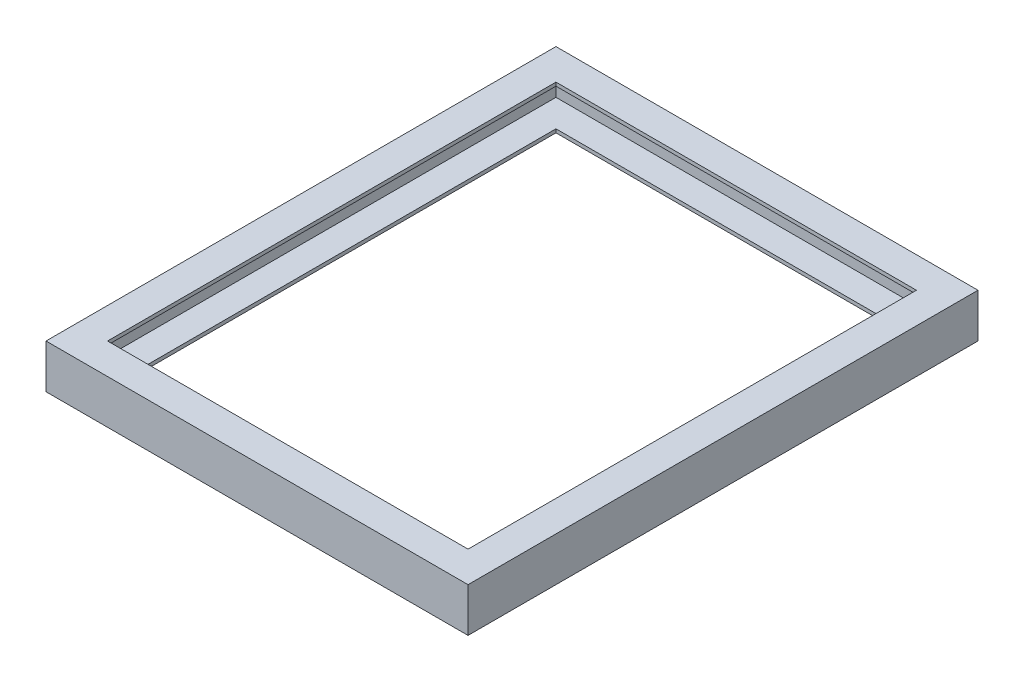
from build123d import *

# Parameters (mm, degrees)
BOSS_EXTRUDE1_DEPTH = 580
BOSS_EXTRUDE2_DEPTH = 472
BOSS_EXTRUDE3_DEPTH = 580


with BuildPart() as part:
    # Sketch1 → Boss-Extrude1 (new body)
    with BuildSketch(Plane.XY):
        Polygon((-10.73531847, 12.748914521), (-45.73531847, 12.748914521), (-45.73531847, -37.251085479), (-10.73531847, -37.251085479), (-10.73531847, -33.251085479), (-41.73531847, -33.251085479), (-41.73531847, 8.748914521), (-10.73531847, 8.748914521), align=None)
    extrude(amount=BOSS_EXTRUDE1_DEPTH)

    # Sketch2 → Boss-Extrude2 (add)
    with BuildSketch(Plane(origin=(-41.73531847, 0, 0), x_dir=(0, 0, -1), z_dir=(1, 0, 0))):
        Polygon((-545, 12.748914521), (-580, 12.748914521), (-580, -37.251085479), (-545, -37.251085479), (-545, -33.251085479), (-576, -33.251085479), (-576, 8.748914521), (-545, 8.748914521), align=None)
        Polygon((-35, -33.251085479), (-35, -37.251085479), (0, -37.251085479), (0, 12.748914521), (-35, 12.748914521), (-35, 8.748914521), (-4, 8.748914521), (-4, -33.251085479), align=None)
    extrude(amount=BOSS_EXTRUDE2_DEPTH)

    # Sketch3 → Boss-Extrude3 (add)
    with BuildSketch(Plane.XY.offset(580)):
        Polygon((399.26468153, 12.748914521), (434.26468153, 12.748914521), (434.26468153, -37.251085479), (399.26468153, -37.251085479), (399.26468153, -33.251085479), (430.26468153, -33.251085479), (430.26468153, 8.748914521), (399.26468153, 8.748914521), align=None)
    extrude(amount=-BOSS_EXTRUDE3_DEPTH)


solid = part.part
